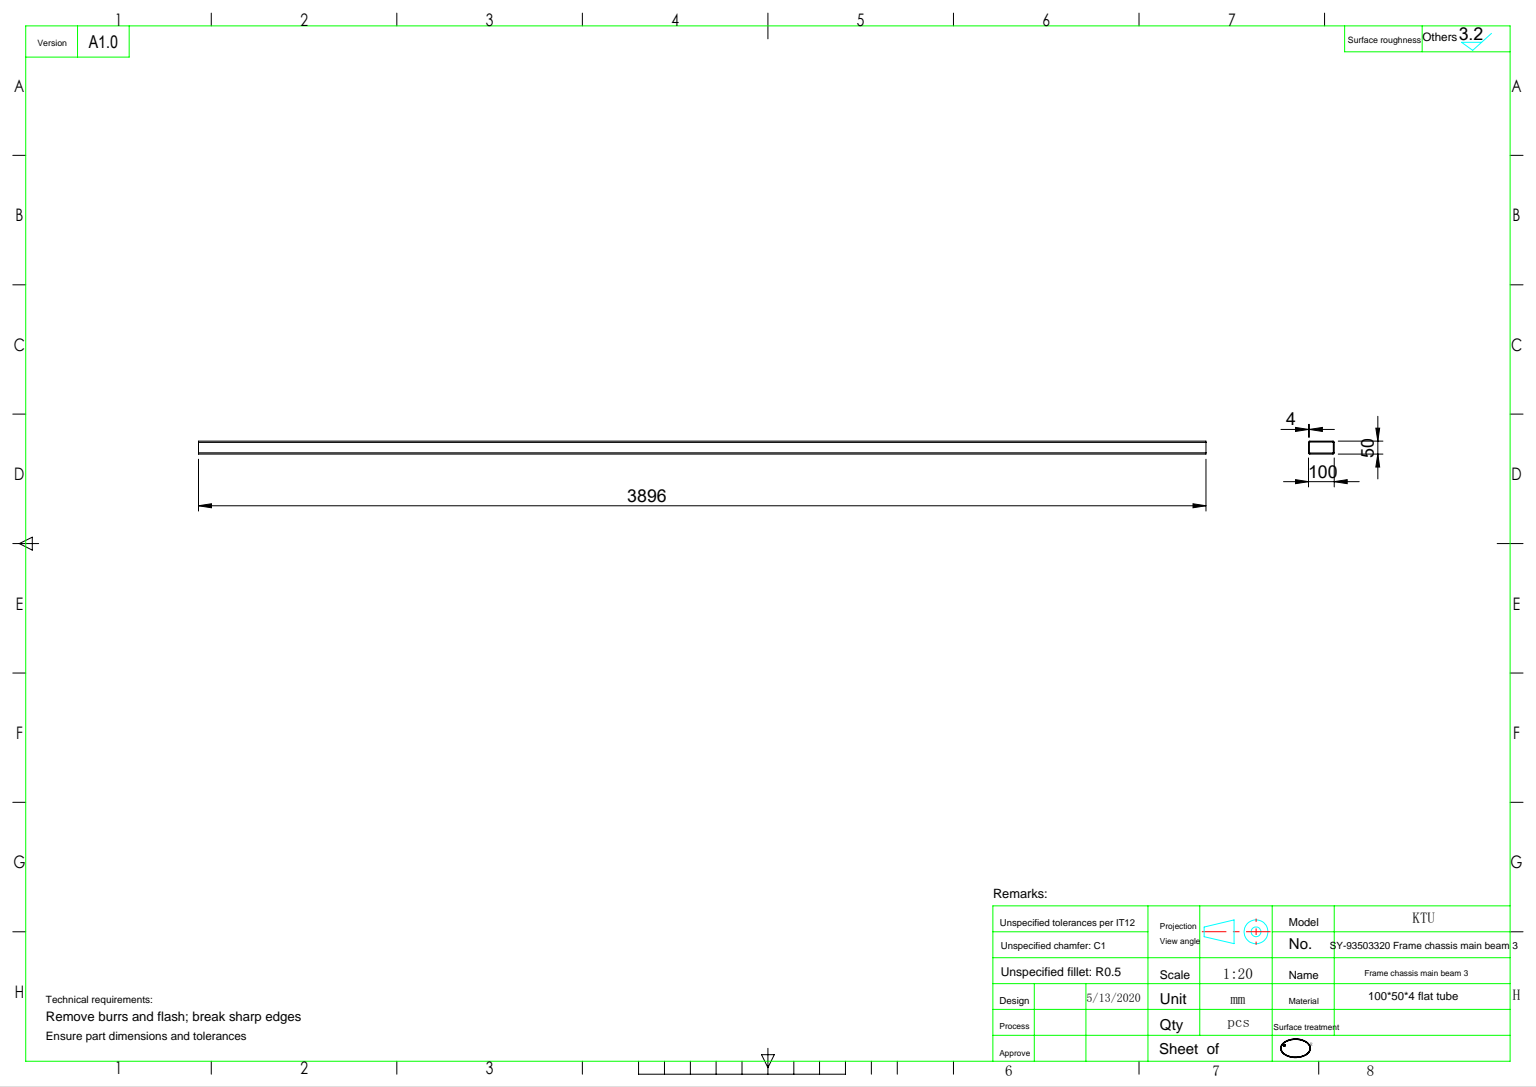
SolidWorks part; units mm, degrees
ref_plane "前视基准面" through (0, 0, 0) normal (0, 0, 1) x (1, 0, 0)
ref_plane "上视基准面" through (0, 0, 0) normal (0, 1, 0) x (1, 0, 0)
ref_plane "右视基准面" through (0, 0, 0) normal (1, 0, 0) x (0, 0, -1)
sketch "草图1" plane through (0, 0, 0) normal (0, 0, 1) x (1, 0, 0)
  line L1 (-45, 25) -> (45, 25)
  line L2 (-50, 20) -> (-50, -20)
  line L3 (-45, -25) -> (45, -25)
  line L4 (50, 20) -> (50, -20)
  line L5 (-50, 25) -> (50, -25) construction
  line L6 (-50, -25) -> (50, 25) construction
  arc A0 (45, -25) -> (50, -20) centre (45, -20) ccw
  arc A1 (45, 25) -> (50, 20) centre (45, 20) cw
  arc A2 (-50, -20) -> (-45, -25) centre (-45, -20) ccw
  arc A3 (-45, 25) -> (-50, 20) centre (-45, 20) ccw
  point P0 (0, 0)
  dimension "D3" = 5
  dimension "D1" = 100
  dimension "D2" = 50
extrude "拉伸-薄壁1" add sketch "草图1" along normal mid plane 3896 thin
